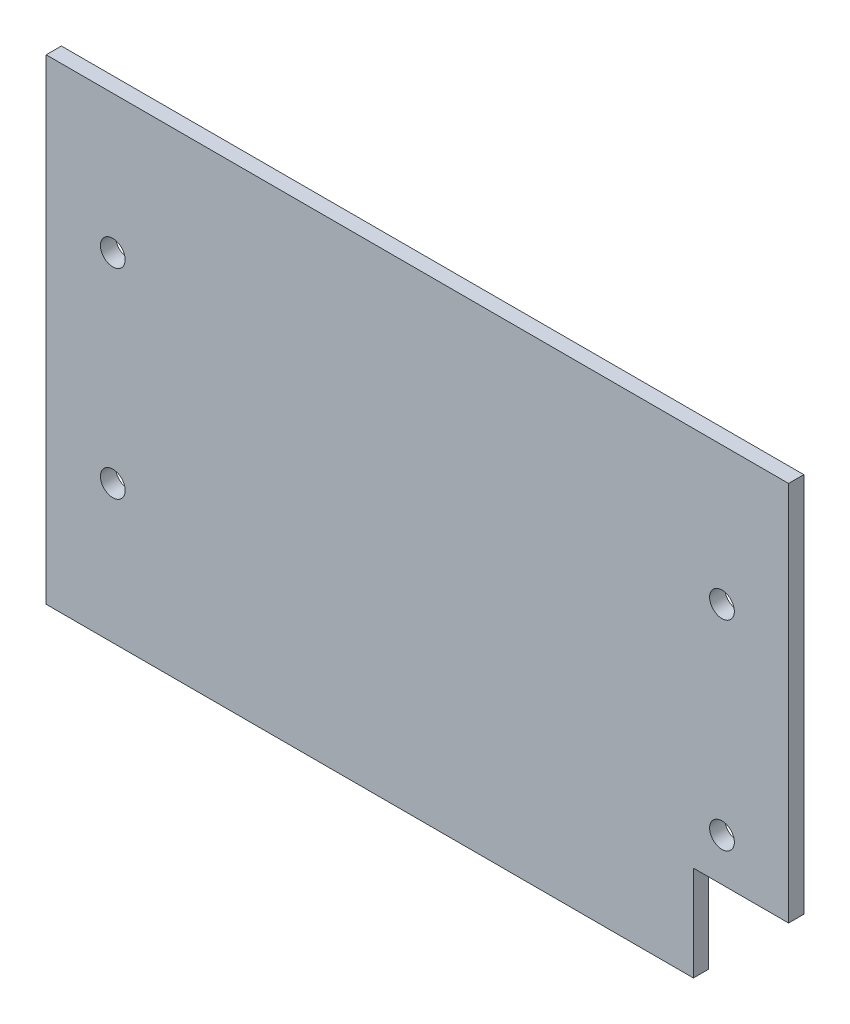
SolidWorks part; units mm, degrees
ref_plane "前视基准面" through (0, 0, 0) normal (0, 0, 1) x (1, 0, 0)
ref_plane "上视基准面" through (0, 0, 0) normal (0, 1, 0) x (1, 0, 0)
ref_plane "右视基准面" through (0, 0, 0) normal (1, 0, 0) x (0, 0, -1)
sketch "草图1" plane through (0, 0, 0) normal (0, 0, 1) x (1, 0, 0)
  line L0 (0, 0) -> (0, 250)
  line L1 (0, 250) -> (390, 250)
  line L2 (390, 250) -> (390, 0)
  line L3 (390, 0) -> (0, 0)
extrude "凸台-拉伸1" add sketch "草图1" along normal blind 8
sketch "草图2" plane through (0, 0, 8) normal (0, 0, 1) x (1, 0, 0)
  line L7 (35, 72.5) -> (355, 72.5)
  line L9 (355, 177.5) -> (355, 72.5)
  line L10 (35, 177.5) -> (355, 177.5)
  line L11 (35, 177.5) -> (35, 72.5)
  circle A0 centre (35, 177.5) radius 6.5
  circle A1 centre (355, 177.5) radius 6.5
  circle A2 centre (355, 72.5) radius 6.5
  circle A3 centre (35, 72.5) radius 6.5
extrude "切除-拉伸1" cut sketch "草图2" against normal blind 8 contours L10 A0 L11 | L11 A0 L10 | L7 A3 L11 | L11 A3 L7 | L7 A2 L9 | L9 A2 L7 | L10 A1 L9 | L9 A1 L10
sketch "草图3" plane through (0, 0, 8) normal (0, 0, 1) x (1, 0, 0)
  line L6 (390, 0) -> (340, 0)
  line L7 (0, 0) -> (390, 0) construction
  line L8 (340, 0) -> (340, 50)
  line L9 (340, 50) -> (390, 50)
  line L10 (390, 0) -> (390, 250) construction
  line L11 (390, 50) -> (390, 0)
extrude "切除-拉伸2" cut sketch "草图3" against normal blind 60
